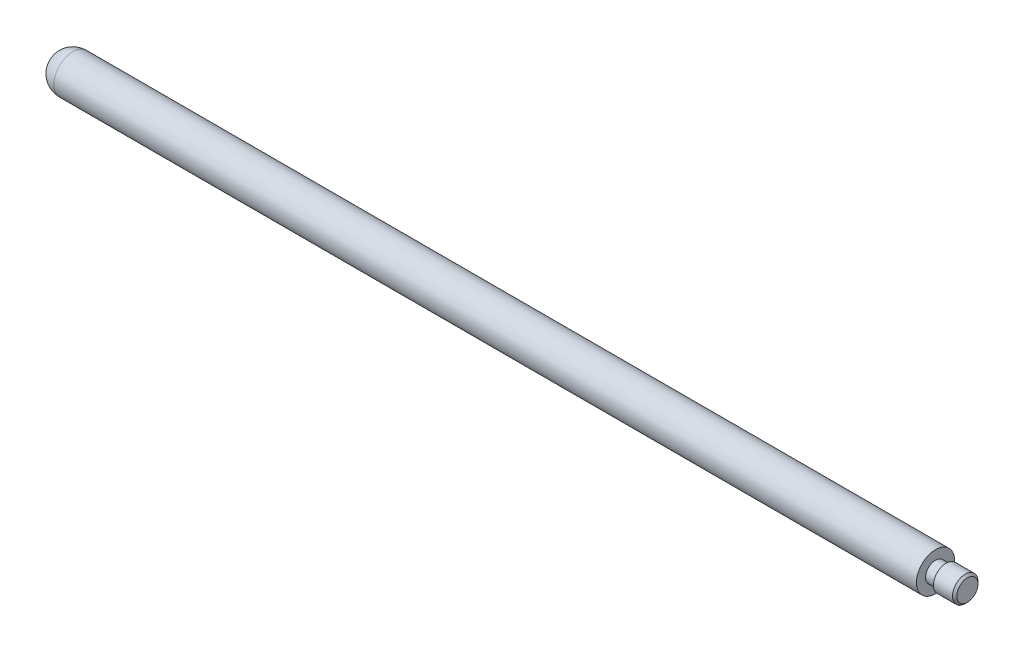
from build123d import *

# Parameters (mm, degrees)
CHAMFER1_SIZE = 1


with BuildPart() as part:
    # Sketch1 → Revolve2 (revolve)
    with BuildSketch(Plane.XY, mode=Mode.PRIVATE) as revolve2_sk:
        with BuildLine():
            Line((0, 0), (-10, 0))
            Line((-10, 0), (-15, 0))
            Line((-15, 0), (-430, 0))
            ThreePointArc((-430, 0), (-427.363961031, 6.363961031), (-421, 9))
            Line((-421, 9), (-15, 9))
            Line((-15, 9), (-15, 4.7))
            Line((-15, 4.7), (-10, 4.7))
            Line((-10, 4.7), (-10, 6))
            Line((-10, 6), (0, 6))
            Line((0, 6), (0, 0))
        make_face()
    revolve(revolve2_sk.sketch.rotate(Axis((-15, 0, 0), (-1, 0, 0)), 90), axis=Axis((-15, 0, 0), (-1, 0, 0)))

    # Chamfer1
    chamfer1_edges = [part.edges().sort_by_distance(p)[0] for p in [
        (0, 0, 6),
    ]]
    chamfer(chamfer1_edges, length=CHAMFER1_SIZE)


solid = part.part
